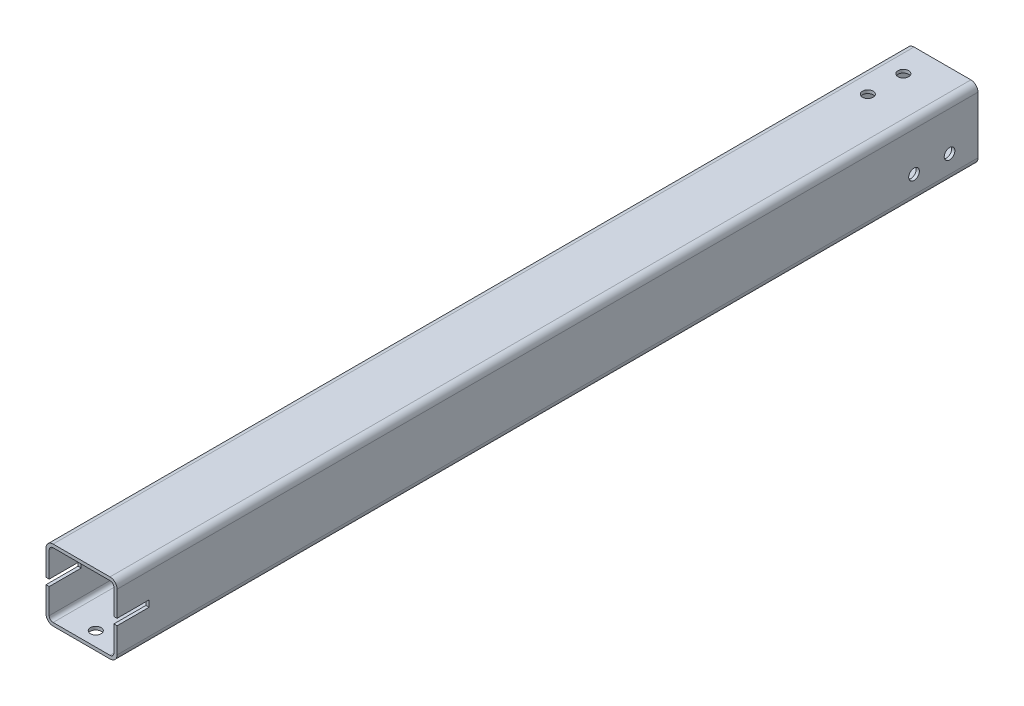
SolidWorks part; units mm, degrees
material "STKR400"
ref_plane "Plane1" through (0, 0, 0) normal (0, 0, 1) x (1, 0, 0)
ref_plane "Plane2" through (0, 0, 0) normal (0, 1, 0) x (1, 0, 0)
ref_plane "Plane3" through (0, 0, 0) normal (1, 0, 0) x (0, 0, -1)
sketch "Sketch1" plane through (0, 0, 0) normal (0, 0, 1) x (1, 0, 0)
  line L0 (-40, -45.5) -> (40, -45.5)
  line L1 (-45.5, -40) -> (-45.5, 40)
  line L2 (40, 45.5) -> (-40, 45.5)
  line L3 (45.5, 40) -> (45.5, -40)
  line L4 (-40, -50) -> (40, -50)
  line L5 (-50, -40) -> (-50, 40)
  line L6 (40, 50) -> (-40, 50)
  line L7 (50, 40) -> (50, -40)
  arc A0 (50, 40) -> (40, 50) centre (40, 40) ccw
  arc A1 (40, -50) -> (50, -40) centre (40, -40) ccw
  arc A2 (-50, -40) -> (-40, -50) centre (-40, -40) ccw
  arc A3 (-40, 50) -> (-50, 40) centre (-40, 40) ccw
  arc A4 (-40, 45.5) -> (-45.5, 40) centre (-40, 40) ccw
  arc A5 (45.5, 40) -> (40, 45.5) centre (40, 40) ccw
  arc A6 (40, -45.5) -> (45.5, -40) centre (40, -40) ccw
  arc A7 (-45.5, -40) -> (-40, -45.5) centre (-40, -40) ccw
  point P0 (-50, 0)
  point P1 (50, 0)
  point P2 (0, 50)
  point P3 (0, -50)
  point P4 (0, 0)
  point P5 (-50, -50)
  point P6 (50, -50)
  point P7 (50, 50)
  point P8 (-50, 50)
extrude "Boss-Extrude1" add sketch "Sketch1" along normal blind 1211
sketch "草图1" plane through (50, 0, 0) normal (1, 0, 0) x (0, 0, -1)
  line L0 (-1211, 50) -> (0, 50) construction
  circle A0 centre (-40, -15) radius 7.5
  circle A1 centre (-90, -15) radius 7.5
  dimension "D1" = 15
  dimension "D2" = 50
  dimension "D3" = 40
  dimension "D4" = 65
extrude "Cut-Extrude1" cut sketch "草图1" against normal up to next
sketch "Sketch2" plane through (0, -50, 0) normal (0, -1, 0) x (1, 0, 0)
  line L0 (-40, 1211) -> (40, 1211) construction
  circle A0 centre (0, 20) radius 7.5
  circle A1 centre (0, 90) radius 7.5
  circle A2 centre (0, 1191) radius 7.5
  dimension "D1" = 15
  dimension "D4" = 70
  dimension "D5" = 20
  dimension "D2" = 50
  dimension "D3" = 20
extrude "Cut-Extrude2" cut sketch "Sketch2" against normal up to next
sketch "Sketch3" plane through (0, 50, 0) normal (0, 1, 0) x (1, 0, 0)
  line L0 (50, -1211) -> (50, 0) construction
  circle A0 centre (-15, -40) radius 7.5
  circle A1 centre (-15, -90) radius 7.5
  dimension "D1" = 15
  dimension "D2" = 40
  dimension "D3" = 50
  dimension "D4" = 65
extrude "Cut-Extrude3" cut sketch "Sketch3" against normal up to next
sketch "Sketch4" plane through (50, 0, 0) normal (1, 0, 0) x (0, 0, -1)
  line L0 (-1211, -40) -> (-1211, 40) construction
  line L1 (-1211, -4.5) -> (-1166, -4.5)
  line L2 (-1211, -4.5) -> (-1211, 4.5)
  line L3 (-1211, 4.5) -> (-1166, 4.5)
  line L4 (-1166, -4.5) -> (-1166, 4.5)
  line L5 (-1211, -50) -> (0, -50) construction
  dimension "D1" = 45.5
  dimension "D2" = 9
  dimension "D3" = 45
extrude "Cut-Extrude4" cut sketch "Sketch4" against normal through all
